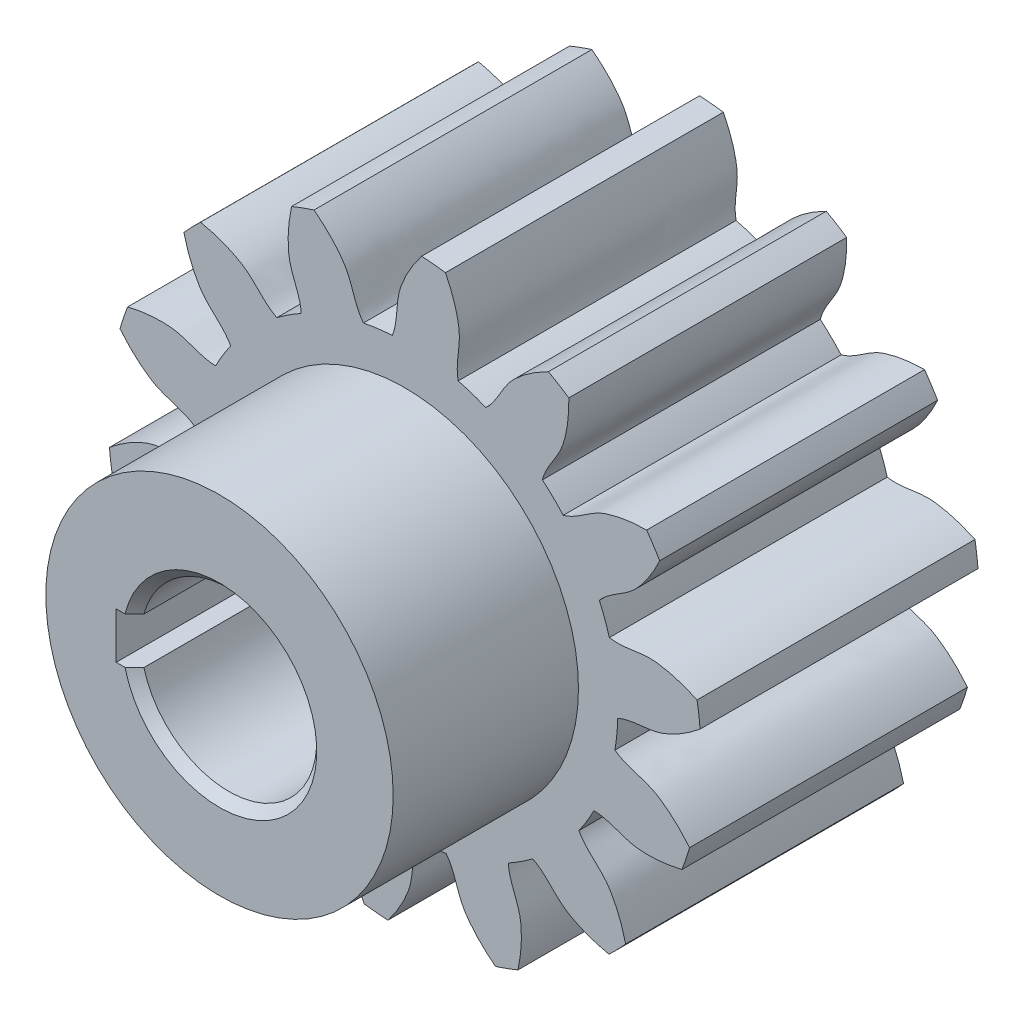
SolidWorks part; units mm, degrees
material "45"
ref_plane "Front Plane" through (0, 0, 0) normal (0, 0, 1) x (1, 0, 0)
ref_plane "Top Plane" through (0, 0, 0) normal (0, 1, 0) x (1, 0, 0)
ref_plane "Right Plane" through (0, 0, 0) normal (1, 0, 0) x (0, 0, -1)
sketch "Sketch1" plane through (0, 0, 0) normal (0, 0, 1) x (1, 0, 0)
  circle A0 centre (0, 0) radius 46
  circle A1 centre (0, 0) radius 19
  dimension "D1" = 38
  dimension "D2" = 92
extrude "Boss-Extrude1" add sketch "Sketch1" along normal blind 60
sketch "Sketch2" plane through (0, 0, 0) normal (0, 0, 1) x (1, 0, 0)
  arc A0 (63.1045, 10.6686) -> (63.7594, 5.5438) centre (0, 0) cw
  arc A1 (44.1675, 12.8542) -> (45.9807, -1.3339) centre (0, 0) cw
  spline S0 degree 3 poles (63.7594, 5.5438) (62.3893, 4.4125) (60.2512, 2.8741) (57.2064, 1.3005) (52.8452, -0.4658) (48.7676, -0.0448) (45.9807, -1.3339) knots 0 0 0 0 0.275475 0.405578 0.530574 1 1 1 1
  spline S1 degree 3 poles (63.1045, 10.6686) (61.494, 11.4189) (59.0377, 12.3702) (55.6949, 13.1275) (51.0297, 13.7402) (47.1891, 12.3074) (44.1675, 12.8542) knots 0 0 0 0 0.275475 0.405578 0.530574 1 1 1 1
extrude "Boss-Extrude2" add sketch "Sketch2" along normal up to surface (60 mm away) up to face at (46, 0, 60)
pattern_circular "CirPattern1" count 14 over 360 about axis through (0, 0, 60) along (0, 0, -1) of "Boss-Extrude2"
sketch "Sketch3" plane through (0, 0, 60) normal (0, 0, 1) x (1, 0, 0)
  circle A0 centre (0, 0) radius 37.5
  circle A1 centre (0, 0) radius 19 construction
  circle A2 centre (0, 0) radius 19
  dimension "D1" = 75
extrude "Boss-Extrude3" add sketch "Sketch3" along normal blind 40
sketch "Sketch4" plane through (0, 0, 0) normal (0, 0, -1) x (-1, 0, 0)
  circle A0 centre (0, 0) radius 27.5
  dimension "D1" = 55
extrude "Cut-Extrude1" cut sketch "Sketch4" against normal blind 22
chamfer "Chamfer1" distance 2 angle 45 1 edges at (19, 0, 100)
sketch "Sketch5" plane through (0, 0, 100) normal (0, 0, 1) x (1, 0, 0)
  line L1 (-15.7, -5) -> (-22.3, -5)
  line L2 (-15.7, -5) -> (-15.7, 5)
  line L3 (-15.7, 5) -> (-22.3, 5)
  line L4 (-22.3, -5) -> (-22.3, 5)
  line L5 (-15.7, -5) -> (-22.3, 5) construction
  line L6 (-15.7, 5) -> (-22.3, -5) construction
  circle A0 centre (0, 0) radius 19 construction
  point P0 (-19, 0)
  dimension "D1" = 10
  dimension "D2" = 41.3
extrude "Cut-Extrude2" cut sketch "Sketch5" against normal up to next
